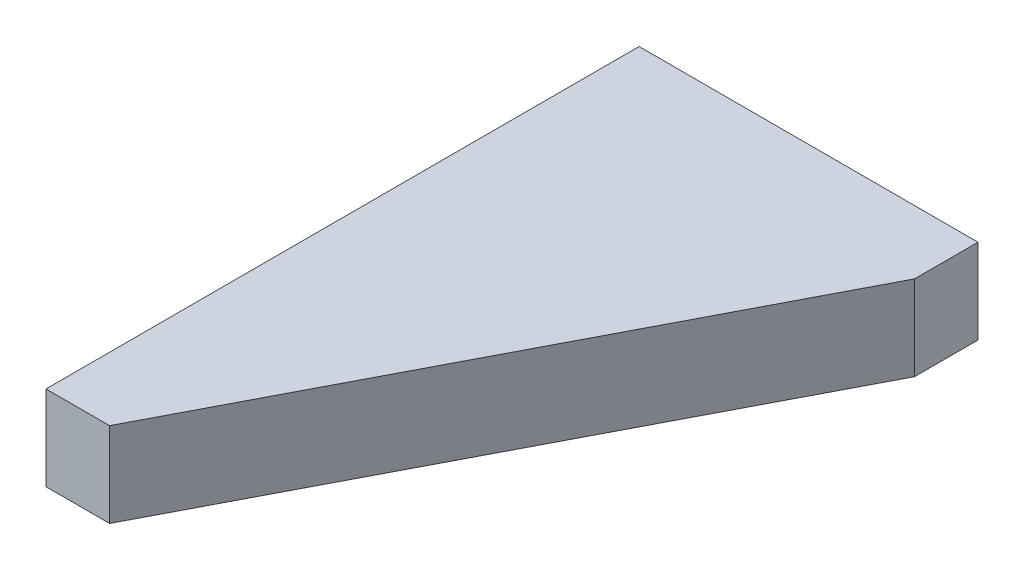
from build123d import *

# Parameters (mm, degrees)
SKETCH_1_W             = 200
SKETCH_1_H             = 140
EXTRUDE_1_DEPTH        = 20
SKETCH_3_OUTSIDE_W     = 250.99
SKETCH_3_OUTSIDE_H     = 190.99
CUT_EXTRUDE_1_DEPTH    = 245.948974278
HOLE_WIZARD_M6_1_D     = 5
HOLE_WIZARD_M6_1_DEPTH = 15
HOLE_WIZARD_M6_1_TIP   = 1.502151548
HOLE_WIZARD_M6_2_D     = 5
HOLE_WIZARD_M6_2_DEPTH = 15
HOLE_WIZARD_M6_2_TIP   = 1.502151548


with BuildPart() as part:
    # 草图1 → 凸台-拉伸1 (new body)
    with BuildSketch(Plane(origin=(0, 0, 0), x_dir=(1, 0, 0), z_dir=(0, 1, 0))):
        with Locations((100, 70)):
            Rectangle(SKETCH_1_W, SKETCH_1_H)
    extrude(amount=EXTRUDE_1_DEPTH)

    # 草图3 outside → 切除-拉伸1 (cut, through all)
    with BuildSketch(Plane(origin=(0, 20, 0), x_dir=(1, 0, 0), z_dir=(0, 1, 0))):
        with Locations((100, 70)):
            Rectangle(SKETCH_3_OUTSIDE_W, SKETCH_3_OUTSIDE_H)
        Polygon((0, 140), (80, 140), (80, 125), (15, 0), (0, 0), align=None, mode=Mode.SUBTRACT)
    extrude(amount=-CUT_EXTRUDE_1_DEPTH, mode=Mode.SUBTRACT)

    # M6 螺纹孔1
    with Locations(Plane.ZY):
        with Locations((-120, 10), (-20, 10)):
            Hole(HOLE_WIZARD_M6_1_D / 2, depth=HOLE_WIZARD_M6_1_DEPTH)
            with Locations((0, 0, -(HOLE_WIZARD_M6_1_DEPTH + HOLE_WIZARD_M6_1_TIP / 2))):  # 118° drill point
                Cone(0, HOLE_WIZARD_M6_1_D / 2, HOLE_WIZARD_M6_1_TIP, mode=Mode.SUBTRACT)

    # M6 螺纹孔2
    with Locations(Plane(origin=(0, 0, -140), x_dir=(-1, 0, 0), z_dir=(0, 0, -1))):
        with Locations((-72.5, 10), (-7.5, 10)):
            Hole(HOLE_WIZARD_M6_2_D / 2, depth=HOLE_WIZARD_M6_2_DEPTH)
            with Locations((0, 0, -(HOLE_WIZARD_M6_2_DEPTH + HOLE_WIZARD_M6_2_TIP / 2))):  # 118° drill point
                Cone(0, HOLE_WIZARD_M6_2_D / 2, HOLE_WIZARD_M6_2_TIP, mode=Mode.SUBTRACT)


solid = part.part
